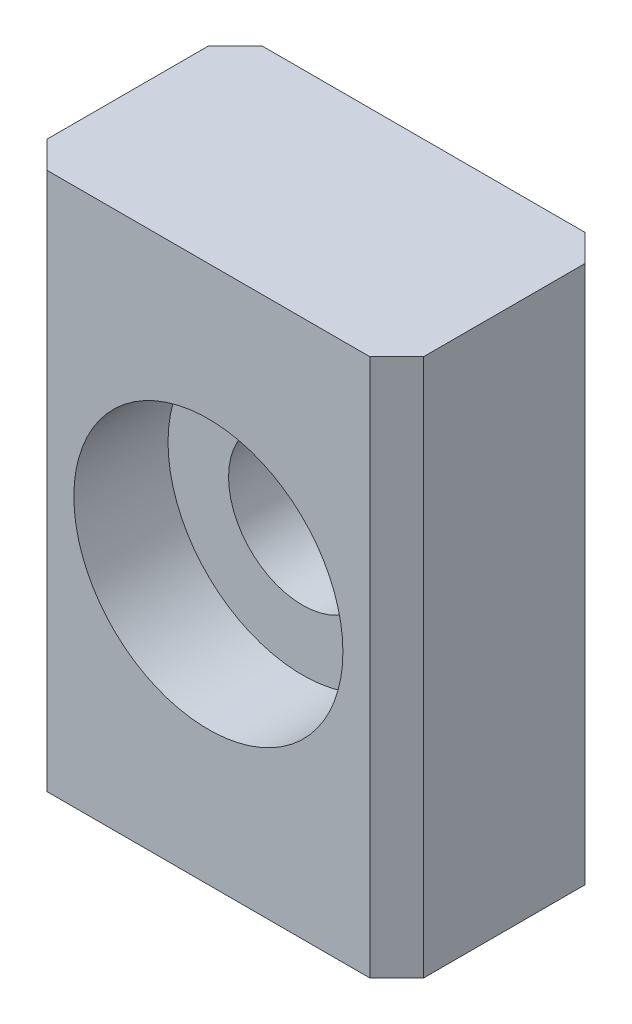
from build123d import *

# Parameters (mm, degrees)
SKETCH1_W          = 14
SKETCH1_H          = 20
BOSS_EXTRUDE_DEPTH = 8
SKETCH2_R          = 5
CUT_EXTRUDE1_DEPTH = 3.5
SKETCH3_R          = 2.75
CUT_EXTRUDE2_DEPTH = 25.824383175
CHAMFER1_SIZE      = 1


with BuildPart() as part:
    # Sketch1 → Boss-Extrude (new body)
    with BuildSketch(Plane.XY):
        with Locations((-7, 10)):
            Rectangle(SKETCH1_W, SKETCH1_H)
    extrude(amount=-BOSS_EXTRUDE_DEPTH)

    # Sketch2 → Cut-Extrude1 (cut)
    with BuildSketch(Plane.XY):
        with Locations((-7, 10)):
            Circle(SKETCH2_R)
    extrude(amount=-CUT_EXTRUDE1_DEPTH, mode=Mode.SUBTRACT)

    # Sketch3 → Cut-Extrude2 (cut, through all)
    with BuildSketch(Plane.XY.offset(-3.5)):
        with Locations((-7, 10)):
            Circle(SKETCH3_R)
    extrude(amount=-CUT_EXTRUDE2_DEPTH, mode=Mode.SUBTRACT)

    # Chamfer1
    chamfer1_edges = [part.edges().sort_by_distance(p)[0] for p in [
        (-14, 10, -8),
        (0, 10, -8),
        (-14, 10, 0),
        (0, 10, 0),
    ]]
    chamfer(chamfer1_edges, length=CHAMFER1_SIZE)


solid = part.part
